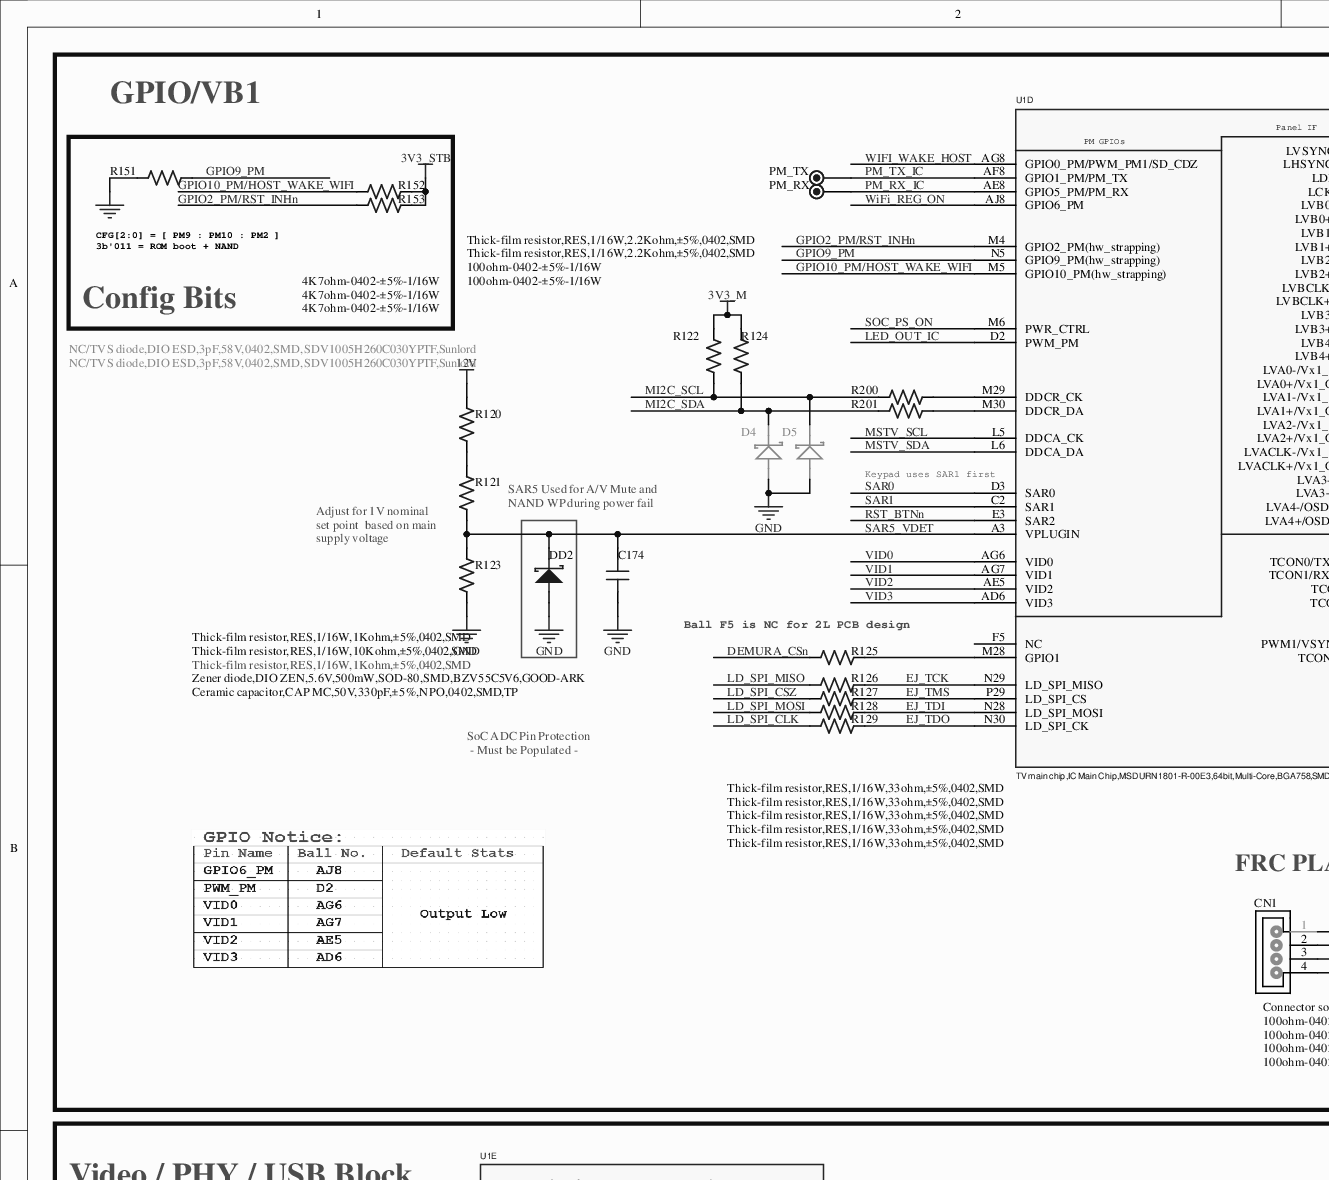
[diagram p0: MISC86290-9.SchDoc, top left]
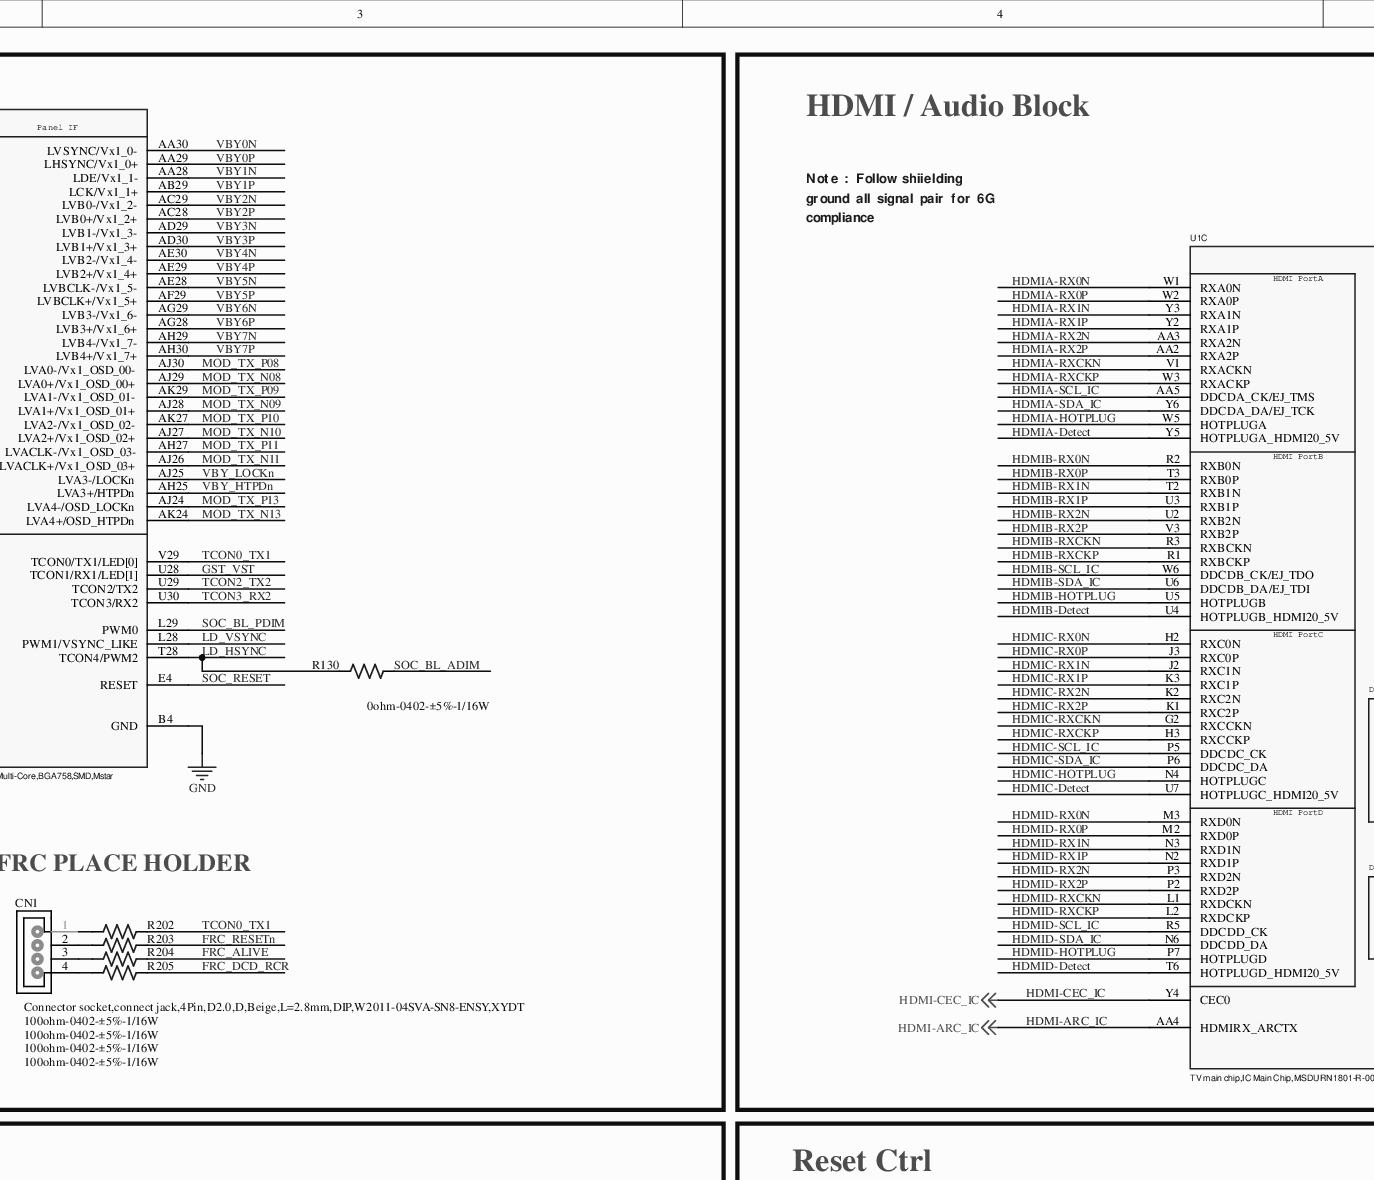
[diagram p1: MISC86290-9.SchDoc, top middle]
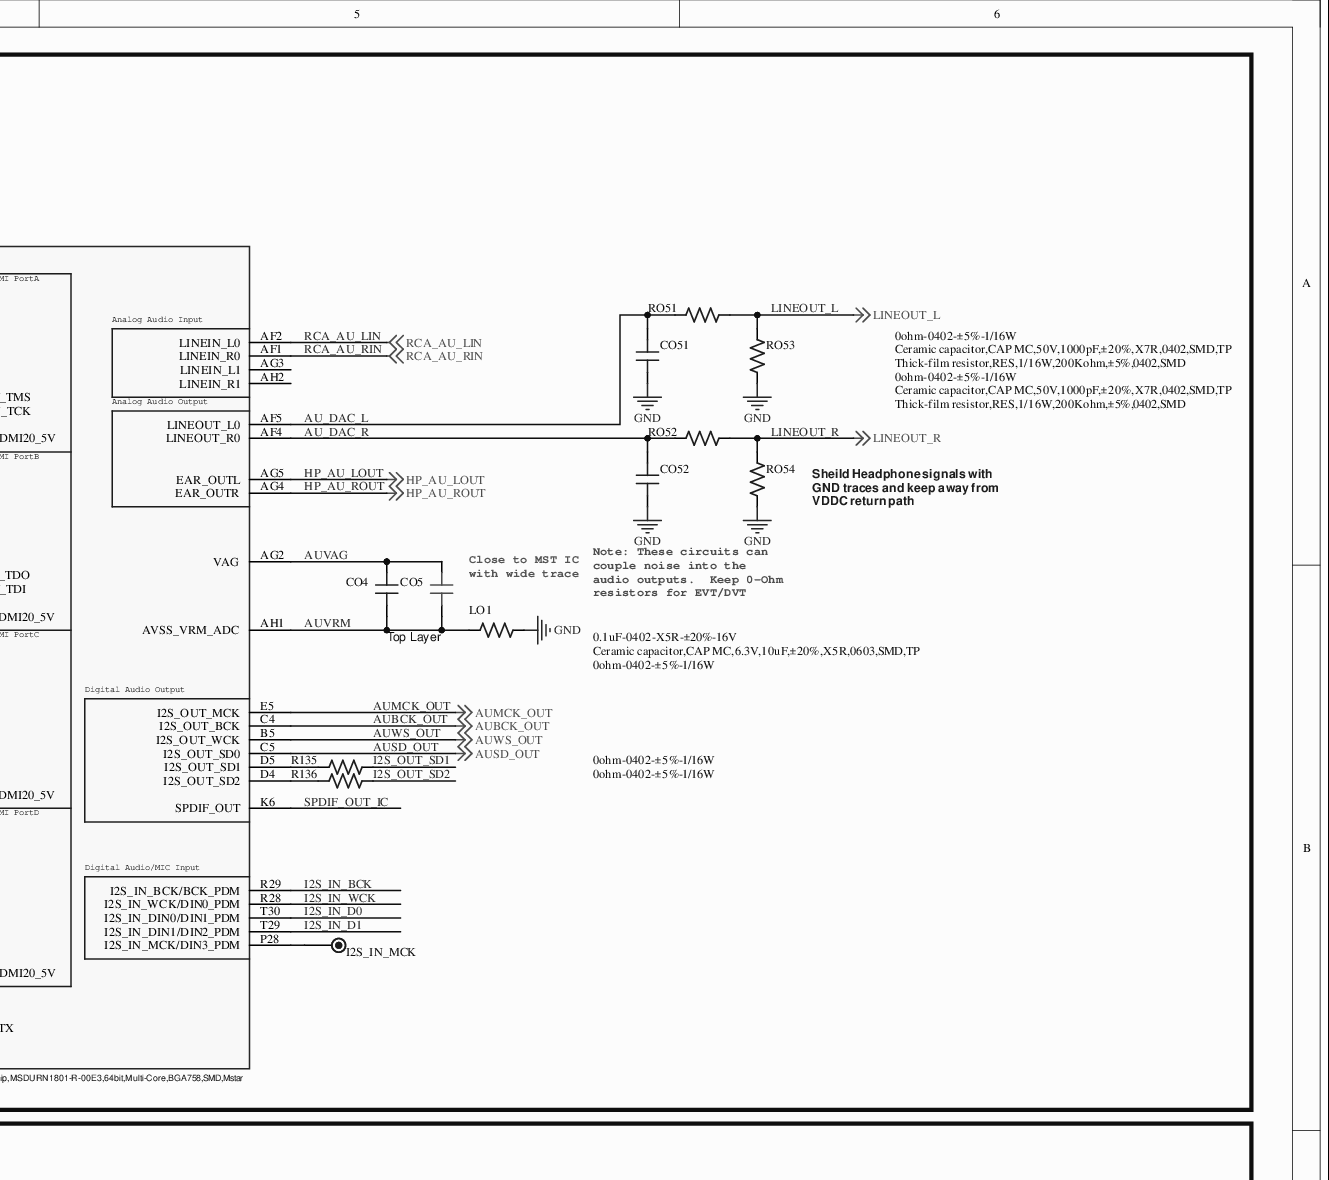
[diagram p2: MISC86290-9.SchDoc, top right]
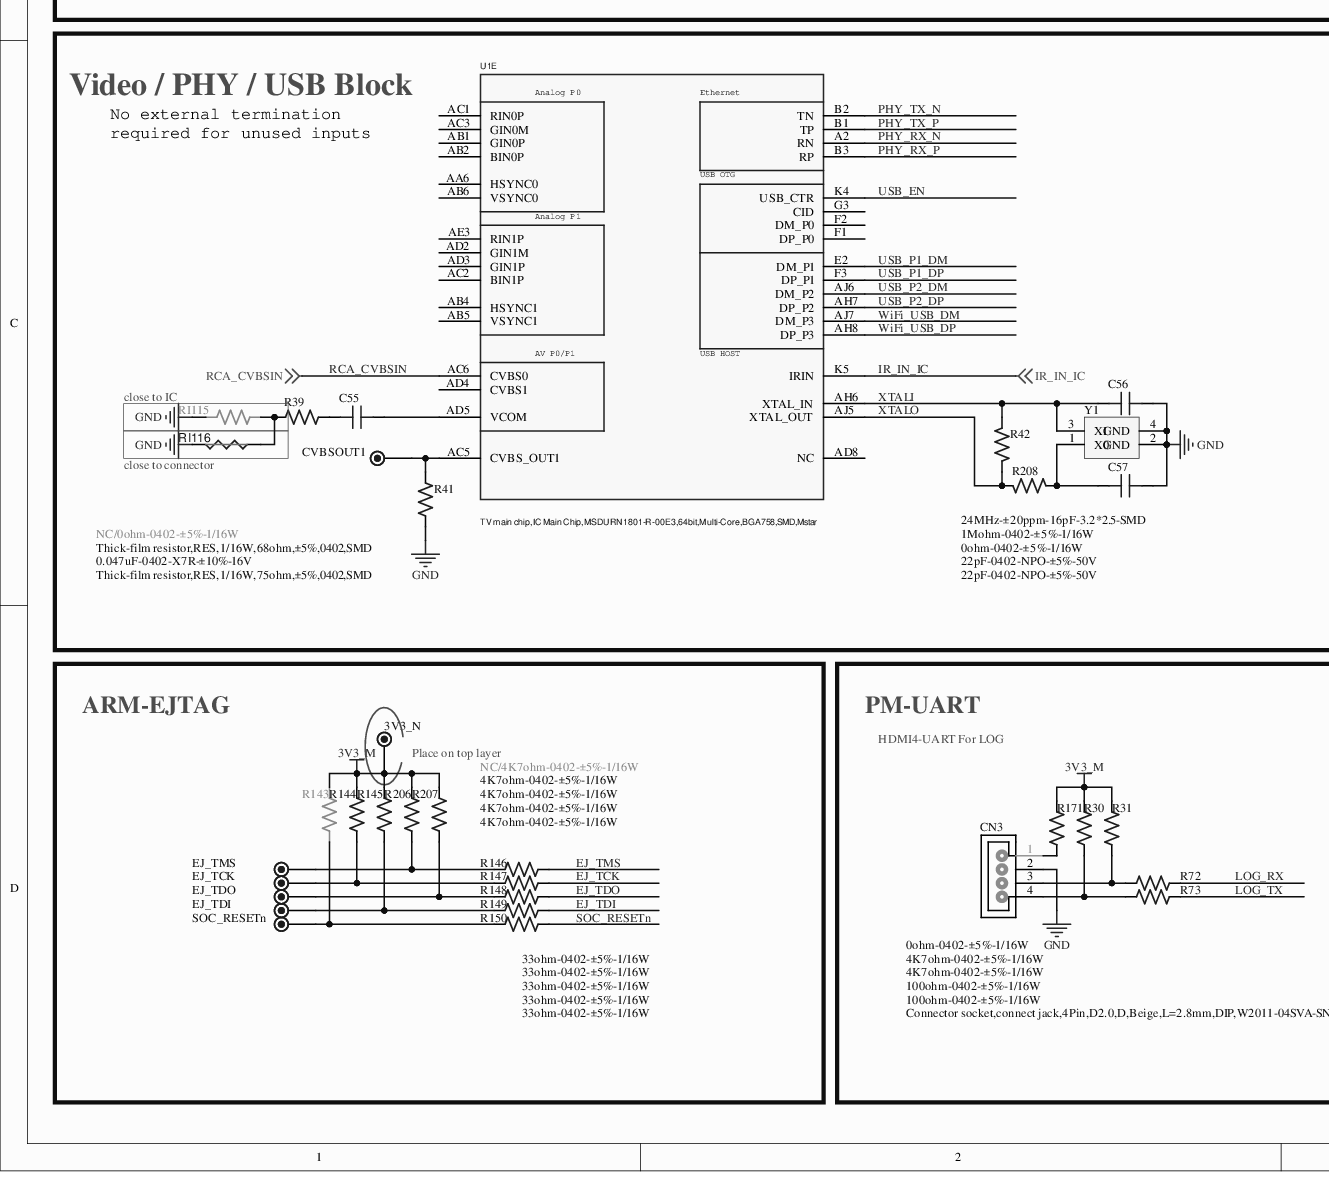
[diagram p3: MISC86290-9.SchDoc, bottom left]
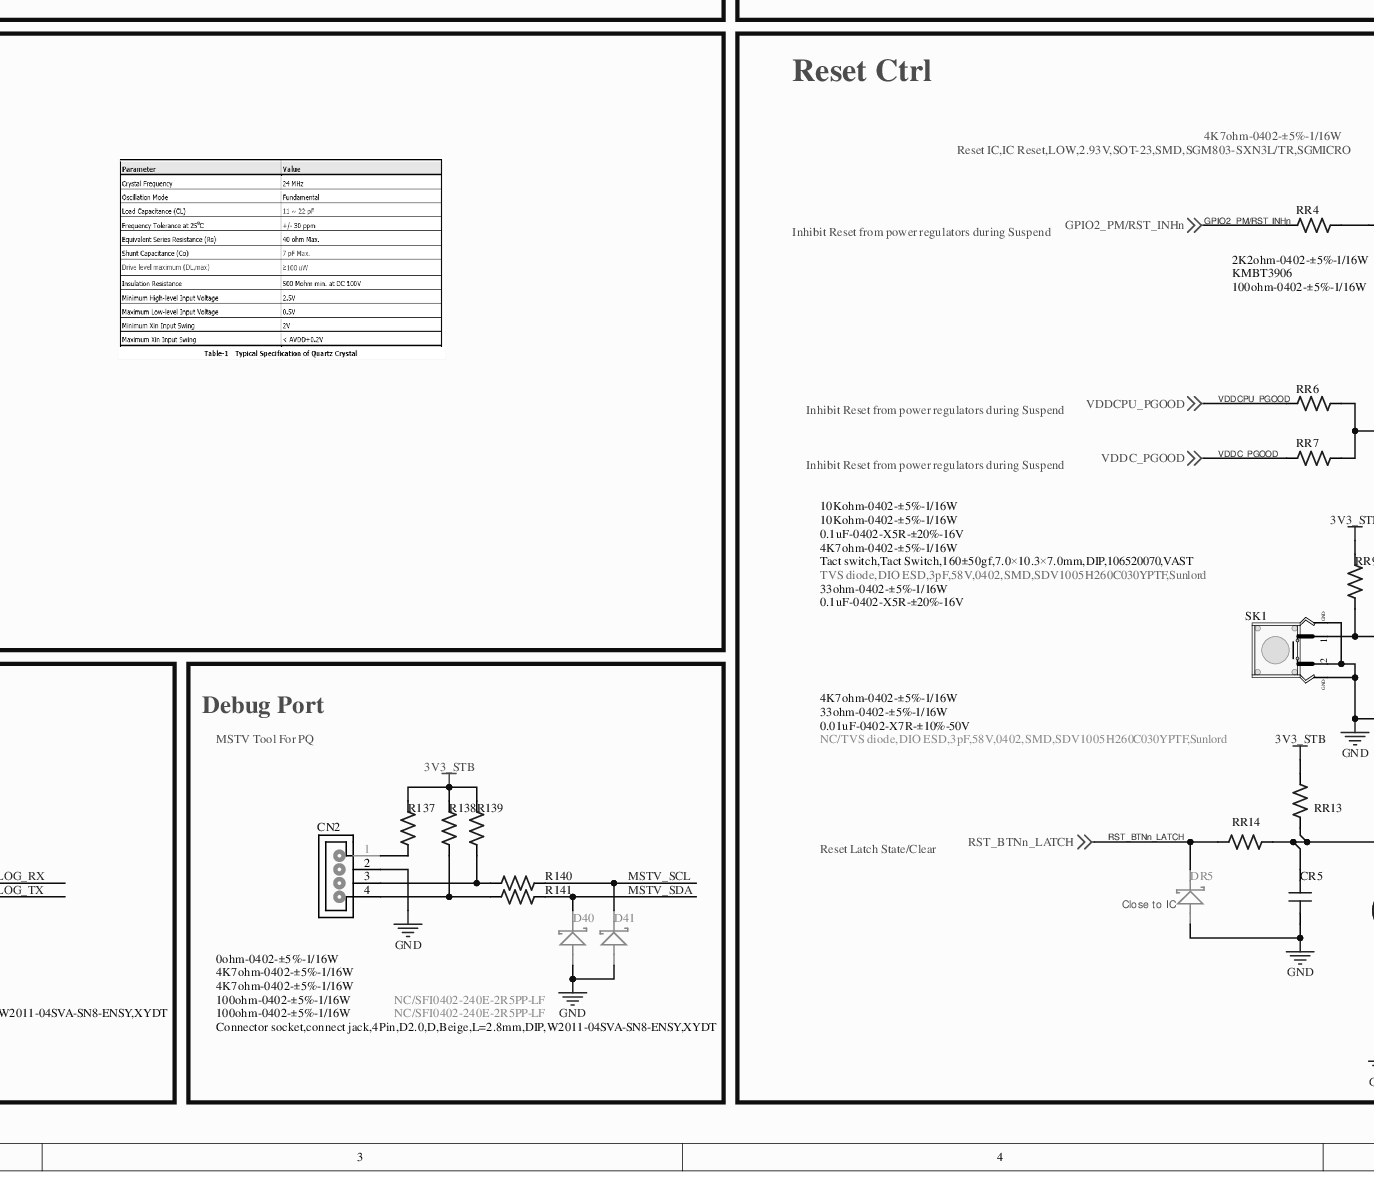
[diagram p4: MISC86290-9.SchDoc, bottom middle]
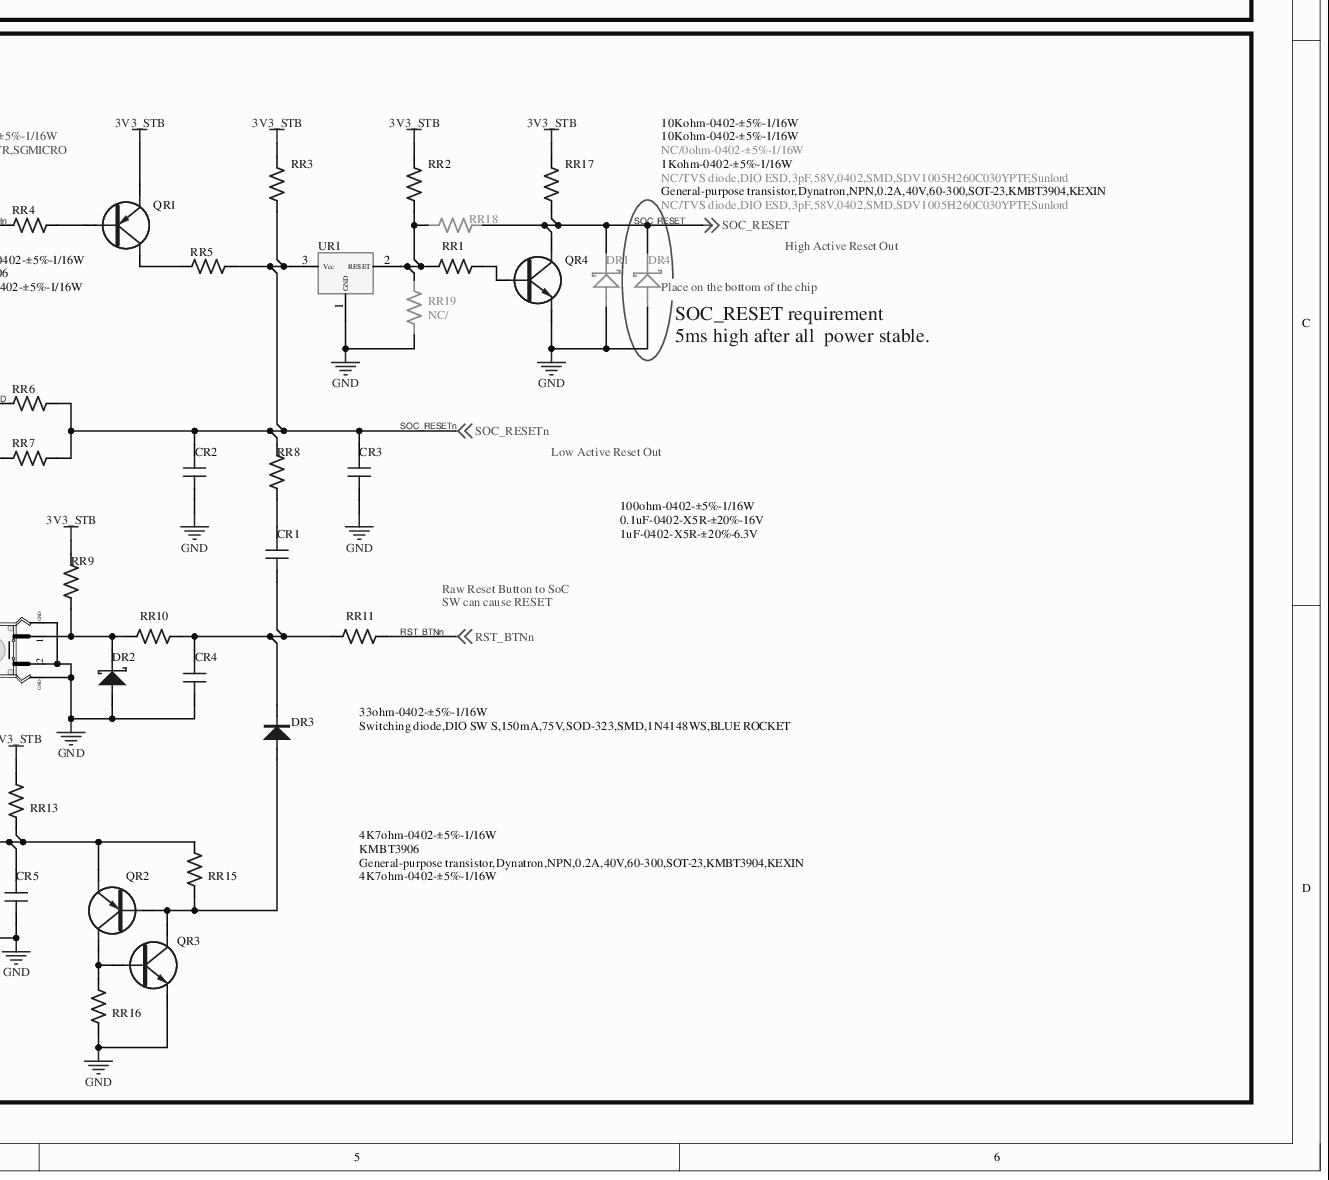
[diagram p5: MISC86290-9.SchDoc, bottom right]
# Altium project MISC86290.PrjPcb (part 7 of 13)

## Sheet MISC86290-9.SchDoc
size 711 x 419 mm

### Parts
3V3_N  TEST  [TP-20]  (value not drawn)
C55  0.047uF-0402-X7R-±10%-16V  [C0402]
C56  22pF-0402-NPO-±5%-50V  [C0402]
C57  22pF-0402-NPO-±5%-50V  [C0402]
C174  Ceramic capacitor,CAP MC,50V,330pF,±5%,NPO,0402,SMD,TP  [C0402]
CN1  Connector socket,connect jack,4Pin,D2.0,D,Beige,L=2.8mm,DIP,W2011-04SVA-SN8-ENSY,XYDT  [SIP4/2.0D-1]
CN2  Connector socket,connect jack,4Pin,D2.0,D,Beige,L=2.8mm,DIP,W2011-04SVA-SN8-ENSY,XYDT  [SIP4/2.0D-1]
CN3  Connector socket,connect jack,4Pin,D2.0,D,Beige,L=2.8mm,DIP,W2011-04SVA-SN8-ENSY,XYDT  [SIP4/2.0D-1]
CO4  0.1uF-0402-X5R-±20%-16V  [C0402]
CO5  Ceramic capacitor,CAP MC,6.3V,10uF,±20%,X5R,0603,SMD,TP  [C0603]
CO51  Ceramic capacitor,CAP MC,50V,1000pF,±20%,X7R,0402,SMD,TP  [C0402]
CO52  Ceramic capacitor,CAP MC,50V,1000pF,±20%,X7R,0402,SMD,TP  [C0402]
CR1  1uF-0402-X5R-±20%-6.3V  [C0402]
CR2  0.1uF-0402-X5R-±20%-16V  [C0402]
CR3  0.1uF-0402-X5R-±20%-16V  [C0402]
CR4  0.1uF-0402-X5R-±20%-16V  [C0402]
CR5  0.01uF-0402-X7R-±10%-50V  [C0402]
CVBSOUT1  TEST  [TP-20]  (value not drawn)
D4  NC/TVS diode,DIO ESD,3pF,58V,0402,SMD,SDV1005H260C030YPTF,Sunlord  [DIODE-S0402]
D5  NC/TVS diode,DIO ESD,3pF,58V,0402,SMD,SDV1005H260C030YPTF,Sunlord  [DIODE-S0402]
D40  NC/SFI0402-240E-2R5PP-LF  [DIODE-S0402]
D41  NC/SFI0402-240E-2R5PP-LF  [DIODE-S0402]
DD2  Zener diode,DIO ZEN,5.6V,500mW,SOD-80,SMD,BZV55C5V6,GOOD-ARK  [DIODE-S0805]
DR1  NC/TVS diode,DIO ESD,3pF,58V,0402,SMD,SDV1005H260C030YPTF,Sunlord  [DIODE-S0402]
DR2  TVS diode,DIO ESD,3pF,58V,0402,SMD,SDV1005H260C030YPTF,Sunlord  [DIODE-S0402]
DR3  Switching diode,DIO SW S,150mA,75V,SOD-323,SMD,1N4148WS,BLUE ROCKET  [DIODE-S-12]
DR4  NC/TVS diode,DIO ESD,3pF,58V,0402,SMD,SDV1005H260C030YPTF,Sunlord  [DIODE-S0402]
DR5  NC/TVS diode,DIO ESD,3pF,58V,0402,SMD,SDV1005H260C030YPTF,Sunlord  [DIODE-S0402]
EJ_TCK  TEST  [TP-20]  (value not drawn)
EJ_TDI  TEST  [TP-20]  (value not drawn)
EJ_TDO  TEST  [TP-20]  (value not drawn)
EJ_TMS  TEST  [TP-20]  (value not drawn)
I2S_IN_MCK  TEST  [TP-20]  (value not drawn)
LO1  0ohm-0402-±5%-1/16W  [R0402]
PM_RX  TEST  [TP-20]  (value not drawn)
PM_TX  TEST  [TP-20]  (value not drawn)
QR1  KMBT3906  [SOT-23]
QR2  KMBT3906  [SOT-23]
QR3  General-purpose transistor,Dynatron,NPN,0.2A,40V,60-300,SOT-23,KMBT3904,KEXIN  [SOT-23]
QR4  General-purpose transistor,Dynatron,NPN,0.2A,40V,60-300,SOT-23,KMBT3904,KEXIN  [SOT-23]
R30  4K7ohm-0402-±5%-1/16W  [R0402]
R31  4K7ohm-0402-±5%-1/16W  [R0402]
R39  Thick-film resistor,RES,1/16W,68ohm,±5%,0402,SMD  [R0402]
R41  Thick-film resistor,RES,1/16W,75ohm,±5%,0402,SMD  [R0402]
R42  1Mohm-0402-±5%-1/16W  [R0402]
R72  100ohm-0402-±5%-1/16W  [R0402]
R73  100ohm-0402-±5%-1/16W  [R0402]
R120  Thick-film resistor,RES,1/16W,1Kohm,±5%,0402,SMD  [R0402]
R121  Thick-film resistor,RES,1/16W,10Kohm,±5%,0402,SMD  [R0402]
R122  Thick-film resistor,RES,1/16W,2.2Kohm,±5%,0402,SMD  [R0402]
R123  Thick-film resistor,RES,1/16W,1Kohm,±5%,0402,SMD  [R0402]
R124  Thick-film resistor,RES,1/16W,2.2Kohm,±5%,0402,SMD  [R0402]
R125  Thick-film resistor,RES,1/16W,33ohm,±5%,0402,SMD  [R0402]
R126  Thick-film resistor,RES,1/16W,33ohm,±5%,0402,SMD  [R0402]
R127  Thick-film resistor,RES,1/16W,33ohm,±5%,0402,SMD  [R0402]
R128  Thick-film resistor,RES,1/16W,33ohm,±5%,0402,SMD  [R0402]
R129  Thick-film resistor,RES,1/16W,33ohm,±5%,0402,SMD  [R0402]
R130  0ohm-0402-±5%-1/16W  [R0402]
R135  0ohm-0402-±5%-1/16W  [R0402]
R136  0ohm-0402-±5%-1/16W  [R0402]
R137  0ohm-0402-±5%-1/16W  [R0402]
R138  4K7ohm-0402-±5%-1/16W  [R0402]
R139  4K7ohm-0402-±5%-1/16W  [R0402]
R140  100ohm-0402-±5%-1/16W  [R0402]
R141  100ohm-0402-±5%-1/16W  [R0402]
R143  NC/4K7ohm-0402-±5%-1/16W  [R0402]
R144  4K7ohm-0402-±5%-1/16W  [R0402]
R145  4K7ohm-0402-±5%-1/16W  [R0402]
R146  33ohm-0402-±5%-1/16W  [R0402]
R147  33ohm-0402-±5%-1/16W  [R0402]
R148  33ohm-0402-±5%-1/16W  [R0402]
R149  33ohm-0402-±5%-1/16W  [R0402]
R150  33ohm-0402-±5%-1/16W  [R0402]
R151  4K7ohm-0402-±5%-1/16W  [R0402]
R152  4K7ohm-0402-±5%-1/16W  [R0402]
R153  4K7ohm-0402-±5%-1/16W  [R0402]
R171  0ohm-0402-±5%-1/16W  [R0402]
R200  100ohm-0402-±5%-1/16W  [R0402]
R201  100ohm-0402-±5%-1/16W  [R0402]
R202  100ohm-0402-±5%-1/16W  [R0402]
R203  100ohm-0402-±5%-1/16W  [R0402]
R204  100ohm-0402-±5%-1/16W  [R0402]
R205  100ohm-0402-±5%-1/16W  [R0402]
R206  4K7ohm-0402-±5%-1/16W  [R0402]
R207  4K7ohm-0402-±5%-1/16W  [R0402]
R208  0ohm-0402-±5%-1/16W  [R0402]
RI115  NC/0ohm-0402-±5%-1/16W  [R0402]
RI116  NC/SHORT  [GND]  (value not drawn)
RO51  0ohm-0402-±5%-1/16W  [R0402]
RO52  0ohm-0402-±5%-1/16W  [R0402]
RO53  Thick-film resistor,RES,1/16W,200Kohm,±5%,0402,SMD  [R0402]
RO54  Thick-film resistor,RES,1/16W,200Kohm,±5%,0402,SMD  [R0402]
RR1  1Kohm-0402-±5%-1/16W  [R0402]
RR2  10Kohm-0402-±5%-1/16W  [R0402]
RR3  4K7ohm-0402-±5%-1/16W  [R0402]
RR4  2K2ohm-0402-±5%-1/16W  [R0402]
RR5  100ohm-0402-±5%-1/16W  [R0402]
RR6  10Kohm-0402-±5%-1/16W  [R0402]
RR7  10Kohm-0402-±5%-1/16W  [R0402]
RR8  100ohm-0402-±5%-1/16W  [R0402]
RR9  4K7ohm-0402-±5%-1/16W  [R0402]
RR10  33ohm-0402-±5%-1/16W  [R0402]
RR11  33ohm-0402-±5%-1/16W  [R0402]
RR13  4K7ohm-0402-±5%-1/16W  [R0402]
RR14  33ohm-0402-±5%-1/16W  [R0402]
RR15  4K7ohm-0402-±5%-1/16W  [R0402]
RR16  4K7ohm-0402-±5%-1/16W  [R0402]
RR17  10Kohm-0402-±5%-1/16W  [R0402]
RR18  NC/0ohm-0402-±5%-1/16W  [R0402]
RR19  NC/  [R0402]
SK1  Tact switch,Tact Switch,160±50gf,7.0×10.3×7.0mm,DIP,106520070,VAST  [KEY-HD-6]
SOC_RESETn  TEST  [TP-20]  (value not drawn)
U1  TV main chip,IC Main Chip,MSDURN1801-R-00E3,64bit,Multi-Core,BGA758,SMD,Mstar  [BGA758/0.65]  (parts C,D,E of 7)
UR1  Reset IC,IC Reset,LOW,2.93V,SOT-23,SMD,SGM803-SXN3L/TR,SGMICRO  [SOT-23-3-1]
Y1  24MHz-±20ppm-16pF-3.2*2.5-SMD  [XTAL-S-3]

### Blocks framed on the sheet
GPIO/VB1: C174 CN1 D4 D5 DD2 PM_RX PM_TX R120-R130 R200-R205 U1
HDMI / Audio Block: CO4 CO5 CO51 CO52 I2S_IN_MCK LO1 R135 R136 RO51-RO54 U1
Config Bits: R151-R153
Video / PHY / USB Block: C55-C57 CVBSOUT1 R39 R41 R42 R208 RI116 U1 Y1
Reset Ctrl: CR1-CR5 DR1-DR5 QR1-QR4 RR1-RR11 RR13-RR19 SK1 UR1
close to IC: RI115
ARM-EJTAG: 3V3_N EJ_TCK EJ_TDI EJ_TDO EJ_TMS R143-R150 R206 R207 SOC_RESETn
PM-UART: CN3 R30 R31 R72 R73 R171
Debug Port: CN2 D40 D41 R137-R141

### Nets
3V3_M: 3V3_N.1 R30.2 R31.2 R122.2 R124.2 R143.2 R144.2 R145.2 R171.2 R206.2 R207.2
3V3_STB: QR1.E R137.2 R138.2 R139.2 R152.1 R153.1 RR2.2 RR3.2 RR9.2 RR13.2 RR17.2
12V: R120.2
GND: C56.2 C57.2 C174.1 CN2.2 CN3.2 CO51.1 CO52.1 CR2.1 CR3.1 CR4.1 CR5.1 D4.A D5.A D40.A D41.A DD2.A DR1.A DR2.A DR4.A DR5.A LO1.2 QR3.E QR4.E R41.1 R123.1 R151.2 RI115.1 RI116.JP_1K RO53.1 RO54.1 RR16.1 RR19.2 SK1.1 SK1.3 SK1.4 U1.B4(GND) UR1.1(GND) Y1.2(GND) Y1.4(GND)
AU_DAC_L: CO51.2 RO51.1 U1.AF5(LINEOUT_L0)
AU_DAC_R: CO52.2 RO52.1 U1.AF4(LINEOUT_R0)
AUBCK_OUT: U1.C4(I2S_OUT_BCK) ; off-sheet AUBCK_OUT
AUMCK_OUT: U1.E5(I2S_OUT_MCK) ; off-sheet AUMCK_OUT
AUSD_OUT: U1.C5(I2S_OUT_SD0) ; off-sheet AUSD_OUT
AUVAG: CO4.2 CO5.2 U1.AG2(VAG)
AUVRM: CO4.1 CO5.1 LO1.1 U1.AH1(AVSS_VRM_ADC)
AUWS_OUT: U1.B5(I2S_OUT_WCK) ; off-sheet AUWS_OUT
DEMURA_CSn: R125.2
EJ_TCK: R126.1 R147.1 U1.N29(LD_SPI_MISO)
EJ_TDI: R128.1 R149.1 U1.N28(LD_SPI_MOSI)
EJ_TDO: R129.1 R148.1 U1.N30(LD_SPI_CK)
EJ_TMS: R127.1 R146.1 U1.P29(LD_SPI_CS)
FRC_ALIVE: R204.2
FRC_DCD_RCR: R205.2
FRC_RESETn: R203.2
GPIO2_PM/RST_INHn: R153.2 RR4.1 U1.M4(GPIO2_PM(hw_strapping)) ; off-sheet GPIO2_PM/RST_INHn
GPIO9_PM: R151.1 U1.N5(GPIO9_PM(hw_strapping))
GPIO10_PM/HOST_WAKE_WIFI: R152.2 U1.M5(GPIO10_PM(hw_strapping))
GST_VST: U1.U28(TCON1/RX1/LED[1])
HDMI-ARC_IC: U1.AA4(HDMIRX_ARCTX) ; off-sheet HDMI-ARC_IC
HDMI-CEC_IC: U1.Y4(CEC0) ; off-sheet HDMI-CEC_IC
HDMIA-Detect: U1.Y5(HOTPLUGA_HDMI20_5V)
HDMIA-HOTPLUG: U1.W5(HOTPLUGA)
HDMIA-RX0N: U1.W1(RXA0N)
HDMIA-RX0P: U1.W2(RXA0P)
HDMIA-RX1N: U1.Y3(RXA1N)
HDMIA-RX1P: U1.Y2(RXA1P)
HDMIA-RX2N: U1.AA3(RXA2N)
HDMIA-RX2P: U1.AA2(RXA2P)
HDMIA-RXCKN: U1.V1(RXACKN)
HDMIA-RXCKP: U1.W3(RXACKP)
HDMIA-SCL_IC: U1.AA5(DDCDA_CK/EJ_TMS)
HDMIA-SDA_IC: U1.Y6(DDCDA_DA/EJ_TCK)
HDMIB-Detect: U1.U4(HOTPLUGB_HDMI20_5V)
HDMIB-HOTPLUG: U1.U5(HOTPLUGB)
HDMIB-RX0N: U1.R2(RXB0N)
HDMIB-RX0P: U1.T3(RXB0P)
HDMIB-RX1N: U1.T2(RXB1N)
HDMIB-RX1P: U1.U3(RXB1P)
HDMIB-RX2N: U1.U2(RXB2N)
HDMIB-RX2P: U1.V3(RXB2P)
HDMIB-RXCKN: U1.R3(RXBCKN)
HDMIB-RXCKP: U1.R1(RXBCKP)
HDMIB-SCL_IC: U1.W6(DDCDB_CK/EJ_TDO)
HDMIB-SDA_IC: U1.U6(DDCDB_DA/EJ_TDI)
HDMIC-Detect: U1.U7(HOTPLUGC_HDMI20_5V)
HDMIC-HOTPLUG: U1.N4(HOTPLUGC)
HDMIC-RX0N: U1.H2(RXC0N)
HDMIC-RX0P: U1.J3(RXC0P)
HDMIC-RX1N: U1.J2(RXC1N)
HDMIC-RX1P: U1.K3(RXC1P)
HDMIC-RX2N: U1.K2(RXC2N)
HDMIC-RX2P: U1.K1(RXC2P)
HDMIC-RXCKN: U1.G2(RXCCKN)
HDMIC-RXCKP: U1.H3(RXCCKP)
HDMIC-SCL_IC: U1.P5(DDCDC_CK)
HDMIC-SDA_IC: U1.P6(DDCDC_DA)
HDMID-Detect: U1.T6(HOTPLUGD_HDMI20_5V)
HDMID-HOTPLUG: U1.P7(HOTPLUGD)
HDMID-RX0N: U1.M3(RXD0N)
HDMID-RX0P: U1.M2(RXD0P)
HDMID-RX1N: U1.N3(RXD1N)
HDMID-RX1P: U1.N2(RXD1P)
HDMID-RX2N: U1.P3(RXD2N)
HDMID-RX2P: U1.P2(RXD2P)
HDMID-RXCKN: U1.L1(RXDCKN)
HDMID-RXCKP: U1.L2(RXDCKP)
HDMID-SCL_IC: U1.R5(DDCDD_CK)
HDMID-SDA_IC: U1.N6(DDCDD_DA)
HP_AU_LOUT: U1.AG5(EAR_OUTL) ; off-sheet HP_AU_LOUT
HP_AU_ROUT: U1.AG4(EAR_OUTR) ; off-sheet HP_AU_ROUT
I2S_IN_BCK: U1.R29(I2S_IN_BCK/BCK_PDM)
I2S_IN_D0: U1.T30(I2S_IN_DIN0/DIN1_PDM)
I2S_IN_D1: U1.T29(I2S_IN_DIN1/DIN2_PDM)
I2S_IN_WCK: U1.R28(I2S_IN_WCK/DIN0_PDM)
I2S_OUT_SD1: R135.2
I2S_OUT_SD2: R136.2
IR_IN_IC: U1.K5(IRIN) ; off-sheet IR_IN_IC
LD_HSYNC: R130.1 U1.T28(TCON4/PWM2)
LD_SPI_CLK: R129.2
LD_SPI_CSZ: R127.2
LD_SPI_MISO: R126.2
LD_SPI_MOSI: R128.2
LD_VSYNC: U1.L28(PWM1/VSYNC_LIKE)
LED_OUT_IC: U1.D2(PWM_PM)
LINEOUT_L: RO51.2 RO53.2 ; off-sheet LINEOUT_L
LINEOUT_R: RO52.2 RO54.2 ; off-sheet LINEOUT_R
LOG_RX: R72.2
LOG_TX: R73.2
MI2C_SCL: D5.K R122.1 R200.1
MI2C_SDA: D4.K R124.1 R201.1
MOD_TX_N08: U1.AJ29(LVA0+/Vx1_OSD_00+)
MOD_TX_N09: U1.AJ28(LVA1+/Vx1_OSD_01+)
MOD_TX_N10: U1.AJ27(LVA2+/Vx1_OSD_02+)
MOD_TX_N11: U1.AJ26(LVACLK+/Vx1_OSD_03+)
MOD_TX_N13: U1.AK24(LVA4+/OSD_HTPDn)
MOD_TX_P08: U1.AJ30(LVA0-/Vx1_OSD_00-)
MOD_TX_P09: U1.AK29(LVA1-/Vx1_OSD_01-)
MOD_TX_P10: U1.AK27(LVA2-/Vx1_OSD_02-)
MOD_TX_P11: U1.AH27(LVACLK-/Vx1_OSD_03-)
MOD_TX_P13: U1.AJ24(LVA4-/OSD_LOCKn)
MSTV_SCL: D41.K R140.2 U1.L5(DDCA_CK)
MSTV_SDA: D40.K R141.2 U1.L6(DDCA_DA)
PHY_RX_N: U1.A2(RN)
PHY_RX_P: U1.B3(RP)
PHY_TX_N: U1.B2(TN)
PHY_TX_P: U1.B1(TP)
PM_RX_IC: PM_RX.1 U1.AE8(GPIO5_PM/PM_RX)
PM_TX_IC: PM_TX.1 U1.AF8(GPIO1_PM/PM_TX)
RCA_AU_LIN: U1.AF2(LINEIN_L0) ; off-sheet RCA_AU_LIN
RCA_AU_RIN: U1.AF1(LINEIN_R0) ; off-sheet RCA_AU_RIN
RCA_CVBSIN: U1.AC6(CVBS0) ; off-sheet RCA_CVBSIN
RST_BTNn: RR11.1 U1.E3(SAR2) ; off-sheet RST_BTNn
RST_BTNn_LATCH: DR5.K RR14.2 ; off-sheet RST_BTNn_LATCH
SAR0: U1.D3(SAR0)
SAR1: U1.C2(SAR1)
SAR5_VDET: C174.2 DD2.K R121.1 R123.2 U1.A3(VPLUGIN)
SOC_BL_ADIM: R130.2
SOC_BL_PDIM: U1.L29(PWM0)
SOC_PS_ON: U1.M6(PWR_CTRL)
SOC_RESET: DR1.K DR4.K QR4.C RR17.1 RR18.2 U1.E4(RESET) ; off-sheet SOC_RESET
SOC_RESETn: CR2.2 CR3.2 R150.1 RR3.1 RR5.1 RR6.1 RR7.1 RR8.2 UR1.3(Vcc) ; off-sheet SOC_RESETn
SPDIF_OUT_IC: U1.K6(SPDIF_OUT)
TCON0_TX1: R202.2 U1.V29(TCON0/TX1/LED[0])
TCON2_TX2: U1.U29(TCON2/TX2)
TCON3_RX2: U1.U30(TCON3/RX2)
USB_EN: U1.K4(USB_CTR)
USB_P1_DM: U1.E2(DM_P1)
USB_P1_DP: U1.F3(DP_P1)
USB_P2_DM: U1.AJ6(DM_P2)
USB_P2_DP: U1.AH7(DP_P2)
VBY0N: U1.AA30(LVSYNC/Vx1_0-)
VBY0P: U1.AA29(LHSYNC/Vx1_0+)
VBY1N: U1.AA28(LDE/Vx1_1-)
VBY1P: U1.AB29(LCK/Vx1_1+)
VBY2N: U1.AC29(LVB0-/Vx1_2-)
VBY2P: U1.AC28(LVB0+/Vx1_2+)
VBY3N: U1.AD29(LVB1-/Vx1_3-)
VBY3P: U1.AD30(LVB1+/Vx1_3+)
VBY4N: U1.AE30(LVB2-/Vx1_4-)
VBY4P: U1.AE29(LVB2+/Vx1_4+)
VBY5N: U1.AE28(LVBCLK-/Vx1_5-)
VBY5P: U1.AF29(LVBCLK+/Vx1_5+)
VBY6N: U1.AG29(LVB3-/Vx1_6-)
VBY6P: U1.AG28(LVB3+/Vx1_6+)
VBY7N: U1.AH29(LVB4-/Vx1_7-)
VBY7P: U1.AH30(LVB4+/Vx1_7+)
VBY_HTPDn: U1.AH25(LVA3+/HTPDn)
VBY_LOCKn: U1.AJ25(LVA3-/LOCKn)
VDDC_PGOOD: RR7.2 ; off-sheet VDDC_PGOOD
VDDCPU_PGOOD: RR6.2 ; off-sheet VDDCPU_PGOOD
VID0: U1.AG6(VID0)
VID1: U1.AG7(VID1)
VID2: U1.AE5(VID2)
VID3: U1.AD6(VID3)
WiFi_REG_ON: U1.AJ8(GPIO6_PM)
WiFi_USB_DM: U1.AJ7(DM_P3)
WiFi_USB_DP: U1.AH8(DP_P3)
WIFI_WAKE_HOST: U1.AG8(GPIO0_PM/PWM_PM1/SD_CDZ)
XTALI: C56.1 R42.1 U1.AH6(XTAL_IN) Y1.3(XI)
XTALO: R42.2 R208.1 U1.AJ5(XTAL_OUT)
NetC55_1: C55.1 R39.2
NetC55_2: C55.2 U1.AD5(VCOM)
NetC57_1: C57.1 R208.2 Y1.1(X0)
NetCN1_1: CN1.1 R202.1
NetCN1_2: CN1.2 R203.1
NetCN1_3: CN1.3 R204.1
NetCN1_4: CN1.4 R205.1
NetCN2_1: CN2.1 R137.1
NetCN2_3: CN2.3 R139.1 R140.1
NetCN2_4: CN2.4 R138.1 R141.1
NetCN3_1: CN3.1 R171.1
NetCN3_3: CN3.3 R31.1 R72.1
NetCN3_4: CN3.4 R30.1 R73.1
NetCR1_1: CR1.1 CR4.2 DR3.K RR10.1 RR11.2
NetCR1_2: CR1.2 RR8.1
NetCR5_2: CR5.2 QR2.E RR13.1 RR14.1 RR15.2
NetCVBSOUT1_1: CVBSOUT1.1 R41.2 U1.AC5(CVBS_OUT1)
NetDR2_K: DR2.K RR9.1 RR10.2 SK1.2
NetDR3_A: DR3.A QR2.B QR3.C RR15.1
NetEJ_TCK_1: EJ_TCK.1 R144.1 R147.2
NetEJ_TDI_1: EJ_TDI.1 R145.1 R149.2
NetEJ_TDO_1: EJ_TDO.1 R148.2 R207.1
NetEJ_TMS_1: EJ_TMS.1 R146.2 R206.1
NetI2S_IN_MCK_1: I2S_IN_MCK.1 U1.P28(I2S_IN_MCK/DIN3_PDM)
NetQR1_B: QR1.B RR4.2
NetQR1_C: QR1.C RR5.2
NetQR2_C: QR2.C QR3.B RR16.2
NetQR4_B: QR4.B RR1.1
NetR39_1: R39.1 RI115.2 RI116.JP_2K
NetR120_1: R120.1 R121.2
NetR125_1: R125.1 U1.M28(GPIO1)
NetR135_1: R135.1 U1.D5(I2S_OUT_SD1)
NetR136_1: R136.1 U1.D4(I2S_OUT_SD2)
NetR143_1: R143.1 R150.2 SOC_RESETn.1
NetR200_2: R200.2 U1.M29(DDCR_CK)
NetR201_2: R201.2 U1.M30(DDCR_DA)
NetRR1_2: RR1.2 RR2.1 RR18.1 RR19.1 UR1.2(RESET)

Not connected (* = marked no-connect by the designer): U1 AA6(HSYNC0)* AB1(GIN0P)* AB2(BIN0P)* AB4(HSYNC1)* AB5(VSYNC1)* AB6(VSYNC0)* AC1(RIN0P)* AC2(BIN1P)* AC3(GIN0M)* AD2(GIN1M)* AD3(GIN1P)* AD4(CVBS1)* AD8(NC)* AE3(RIN1P)* AG3(LINEIN_L1)* AH2(LINEIN_R1)* F1(DP_P0)* F2(DM_P0)* F5(NC)* G3(CID)*

### Notes on the sheet
- CFG[2:0] = [ PM9 : PM10 : PM2 ]
  3b'011 = ROM boot + NAND
- (near U1) Note : Follow shiielding
  ground all signal pair for 6G
  compliance
- Keypad uses SAR1 first
- Adjust for 1V nominal
  set point  based on main
  supply voltage
- SAR5 Used for A/V Mute and
  NAND WP during power fail
- Sheild Headphone signals with
  GND traces and keep away from
  VDDC return path
- (near R125) Ball F5 is NC for 2L PCB design
- Top Layer
- Close to MST IC
  with wide trace
- Note: These circuits can
  couple noise into the
  audio outputs.  Keep 0-Ohm
  resistors for EVT/DVT
- SoC ADC Pin Protection
  - Must be Populated -
- FRC PLACE HOLDER
- No external termination
  required for unused inputs
- Inhibit Reset from power regulators during Suspend
- (near DR4) Place on the bottom of the chip
- High Active Reset Out
- (near DR4) SOC_RESET requirement
  5ms high after all  power stable.
- (near RI116) close to connector
- Low Active Reset Out
- Raw Reset Button to SoC
- SW can cause RESET
- Place on top layer
- HDMI4-UART For LOG
- MSTV Tool For PQ
- Reset Latch State/Clear
- (near DR5) Close to IC

### Library data of the parts
C55 = 004.003.0000562-D: Ceramic capacitor,CAP MC,16V,0.047uF,±10%,X7R,0402,SMD,TP-D
C56 C57 = 33pF-0402-NPO-±5%-50V-D
C174 CO4 = 004.003.0000505-D: Ceramic capacitor,CAP MC,16V,0.01uF,±10%,X7R,0402,SMD,TP-D
CN1-CN3 = 4PIN-2.0-D-H-G-LD-DHMI
CO5 = 004.003.0000383-D: Ceramic capacitor,CAP MC,6.3V,10uF,±20%,X5R,0603,SMD,TP-D
CO51 CO52 = 004.003.0000503-D: Ceramic capacitor,CAP MC,50V,1000pF,±10%,X7R,0402,SMD,TP-D
CR1 = 1uF-0402-X5R-±20%-6.3V-D
CR2-CR4 = 0.1uF-0402-X5R-±20%-16V-D
CR5 = 0.01uF-0402-X7R-±10%-50V-D
D4 D5 D40 D41 DR1 DR2 DR4 DR5 = AVLC18S02003-D
DD2 = 5.6V-LL-34-1/2W-D
DR3 = 1N4148WS-D
LO1 R130 R135-R137 R171 RI115 RO51 RO52 RR18 = 0ohm-0402-±5%-1/16W-D
QR1 QR2 = LMBT3906LT1G-D-PNP
QR3 = LMBT3904LT1G-D-NPN: Q-NPN-#-#-#
QR4 = KMBT3904-D
R30 R31 R138 R139 R151-R153 RR3 RR9 RR13 RR15 RR16 = 4K7ohm-0402-±5%-1/16W-D
R39 = 004.002.0000721-D: Thick-film resistor,RES,1/16W,68ohm,±5%,0402,SMD-D
R41 = 004.002.0000728-D: Thick-film resistor,RES,1/16W,75ohm,±5%,0402,SMD-D
R42 R208 = 1Mohm-0402-±5%-1/16W-D
R72 R73 R140 R141 RR5 RR8 = 100ohm-0402-±5%-1/16W-D
R120 = 004.002.0000572-D: Thick-film resistor,RES,1/16W,1Kohm,±5%,0402,SMD-D
R121 R123 = 004.002.0000577-D: Thick-film resistor,RES,1/16W,10Kohm,±5%,0402,SMD-D
R122 R124 = 004.002.0000630-D: Thick-film resistor,RES,1/16W,2.2Kohm,±5%,0402,SMD-D
R125-R129 = 004.002.0000658-D: Thick-film resistor,RES,1/16W,33ohm,±5%,0402,SMD-D
R143-R145 R206 R207 RR1 = 1Kohm-0402-±5%-1/16W-D
R146-R150 RR10 RR11 RR14 = 33ohm-0402-±5%-1/16W-D
R200-R205 RR19 = 100Kohm-0402-±5%-1/16W-D
RI116 = GND: Manufacturer: Panasonic; Part Number: ERJ3GEYJ473V; Right: 20; Bottom: 30; CLASS: Discrete; Comments: Digikey
RO53 RO54 = 004.002.0000624-D: Thick-film resistor,RES,1/16W,200Kohm,±5%,0402,SMD-D
RR2 RR6 RR7 RR17 = 10Kohm-0402-±5%-1/16W-D
RR4 = 2K2ohm-0402-±5%-1/16W-D
SK1 = 轻触开关,Tact Switch,160±50gf,7.0×10.3×7.0mm,DIP,KFC-A06-E-4-7.5/4(R),YK-DLMI
U1 = 004.016.0001110-D: TV main chip,IC Main Chip,MSDURN1801-Z1,64bit,Multi-Core,BGA758,SMD,Mstar-D
UR1 = SGM809-SXN3-D
Y1 = 16.000MHz±20PPM-10PF-SMD3225-D: NC: GPS; PCB DECAL: TCXO_3225; Source_Path: EM_66_V2.0_201209181010.DSN; Value: 26M/0.5PPM/1.8V